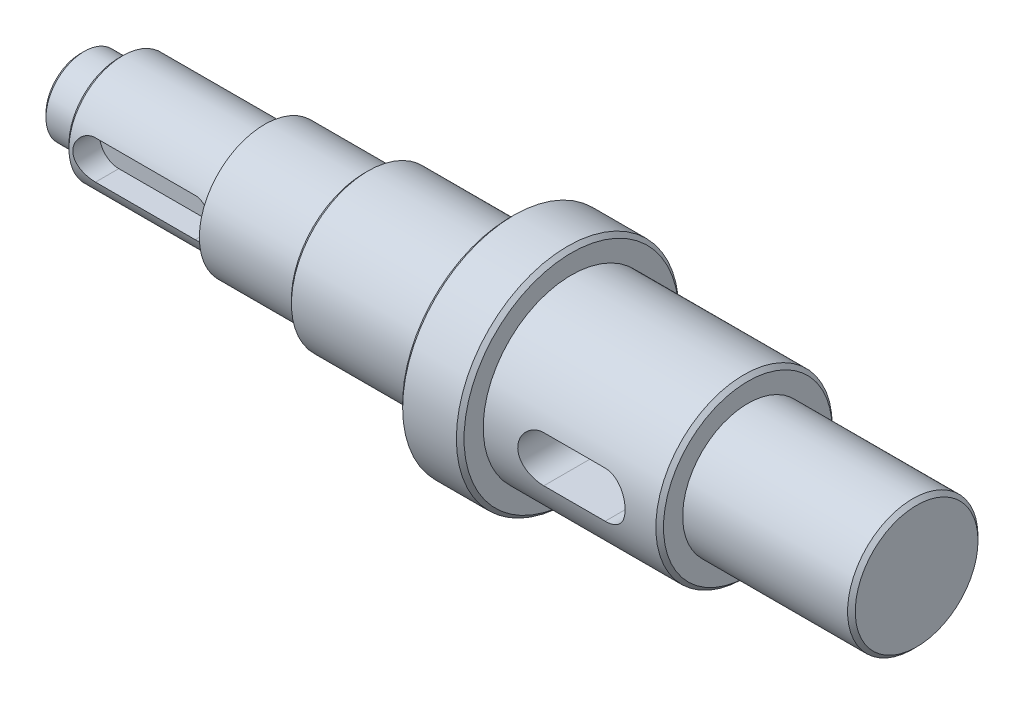
SolidWorks part; units mm, degrees
ref_plane "Front Plane" through (0, 0, 0) normal (0, 0, 1) x (1, 0, 0)
ref_plane "Top Plane" through (0, 0, 0) normal (0, 1, 0) x (1, 0, 0)
ref_plane "Right Plane" through (0, 0, 0) normal (1, 0, 0) x (0, 0, -1)
other "Configuration Table"
sketch "Sketch1" plane through (0, 0, 0) normal (1, 0, 0) x (0, 0, -1)
  circle A0 centre (0, 0) radius 5
  dimension "D1" = 10
extrude "Boss-Extrude1" add sketch "Sketch1" along normal blind 5
sketch "Sketch2" plane through (5, 0, 0) normal (1, 0, 0) x (0, 0, -1)
  circle A0 centre (0, 0) radius 7
  dimension "D1" = 14
extrude "Boss-Extrude2" add sketch "Sketch2" along normal blind 19
sketch "Sketch3" plane through (24, 0, 0) normal (1, 0, 0) x (0, 0, -1)
  circle A0 centre (0, 0) radius 8.5
  dimension "D1" = 17
extrude "Boss-Extrude3" add sketch "Sketch3" along normal blind 13
sketch "Sketch4" plane through (37, 0, 0) normal (1, 0, 0) x (0, 0, -1)
  circle A0 centre (0, 0) radius 10
  dimension "D1" = 20
extrude "Boss-Extrude4" add sketch "Sketch4" along normal blind 19
sketch "Sketch5" plane through (56, 0, 0) normal (1, 0, 0) x (0, 0, -1)
  circle A0 centre (0, 0) radius 14.5
  dimension "D1" = 29
extrude "Boss-Extrude5" add sketch "Sketch5" along normal blind 8
sketch "Sketch6" plane through (64, 0, 0) normal (1, 0, 0) x (0, 0, -1)
  circle A0 centre (0, 0) radius 11.5
  dimension "D1" = 23
extrude "Boss-Extrude6" add sketch "Sketch6" along normal blind 23
sketch "Sketch7" plane through (87, 0, 0) normal (1, 0, 0) x (0, 0, -1)
  circle A0 centre (0, 0) radius 8.5
  dimension "D1" = 17
extrude "Boss-Extrude7" add sketch "Sketch7" along normal blind 22
chamfer "Chamfer1" distance 0.5 angle 45 7 edges at (0, 0, -5) (109, 0, -8.5) (87, 0, -11.5) (64, 0, -14.5) (56, 0, -14.5) (37, 0, -10) (5, 0, -7)
sketch "Sketch8" plane through (0, 0, 0) normal (0, 0, 1) x (1, 0, 0)
  line L0 (8.5, 0) -> (21.5, 0) construction
  line L1 (8.5, 2.5) -> (21.5, 2.5)
  line L2 (8.5, -2.5) -> (21.5, -2.5)
  line L3 (5, 5) -> (5, -5) construction
  arc A0 (8.5, 2.5) -> (8.5, -2.5) centre (8.5, 0) ccw
  arc A1 (21.5, -2.5) -> (21.5, 2.5) centre (21.5, 0) ccw
  point P3 (15, 0)
  point P8 (24, 0)
  point P9 (6, 0)
  dimension "D3" = 2.5
  dimension "D1" = 18
  dimension "D2" = 1
extrude "Cut-Extrude2" cut sketch "Sketch8" against normal blind 3.5 from offset 7
sketch "Sketch9" plane through (0, 0, 0) normal (0, 0, 1) x (1, 0, 0)
  line L0 (71.5, 0) -> (79.5, 0) construction
  line L1 (71.5, 3) -> (79.5, 3)
  line L2 (71.5, -3) -> (79.5, -3)
  line L3 (87, -8.5) -> (87, 8.5) construction
  arc A0 (71.5, 3) -> (71.5, -3) centre (71.5, 0) ccw
  arc A1 (79.5, -3) -> (79.5, 3) centre (79.5, 0) ccw
  point P3 (75.5, 0)
  point P8 (82.5, 0)
  dimension "D3" = 3
  dimension "D1" = 8
  dimension "D2" = 4.5
extrude "Cut-Extrude3" cut sketch "Sketch9" against normal blind 6.5 from offset 11.5
fillet "Fillet1" radius 2 1 edges at (56, 0, -10)
